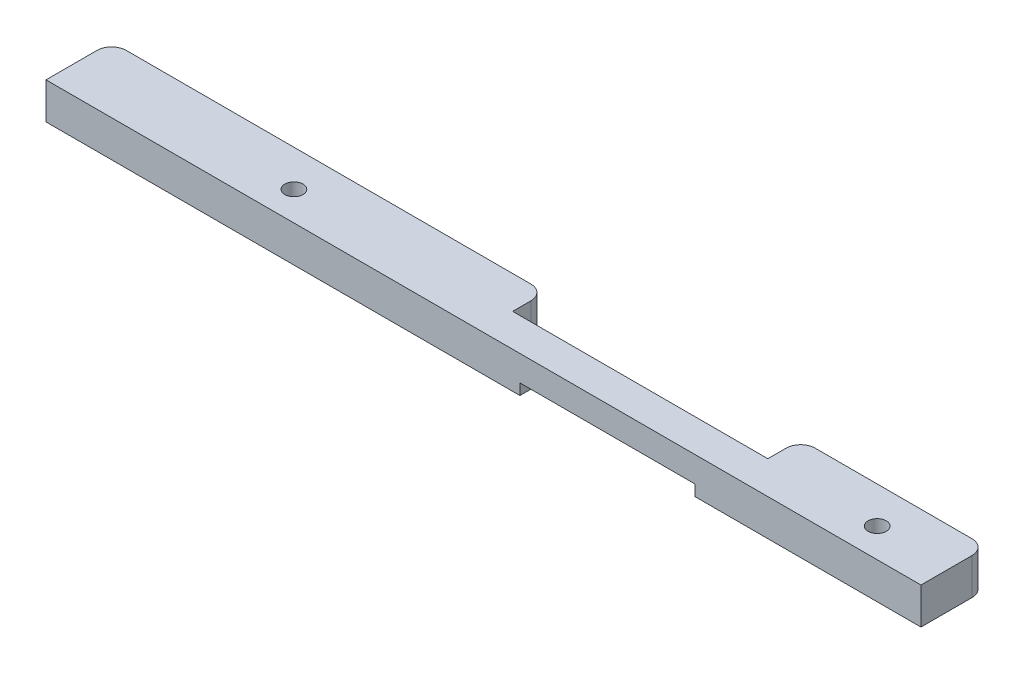
from build123d import *

# Parameters (mm, degrees)
SKETCH1_W             = 120
SKETCH1_H             = 9
BOSS_EXTRUDE1_DEPTH   = 5
M3_TAPPED_HOLE1_D     = 2.5
M3_TAPPED_HOLE1_DEPTH = 8.5
FILLET1_R             = 2
SKETCH4_W             = 35
SKETCH4_H             = 4.5
CUT_EXTRUDE1_DEPTH    = 121.440856855
FILLET2_R             = 2
SKETCH5_W             = 24
SKETCH5_H             = 9
CUT_EXTRUDE2_DEPTH    = 1.5


with BuildPart() as part:
    # Sketch1 → Boss-Extrude1 (new body)
    with BuildSketch(Plane(origin=(0, 0, 0), x_dir=(1, 0, 0), z_dir=(0, 1, 0))):
        with Locations((60, 4.5)):
            Rectangle(SKETCH1_W, SKETCH1_H)
    extrude(amount=BOSS_EXTRUDE1_DEPTH)

    # M3 Tapped Hole1
    with Locations(Plane(origin=(0, 5, 0), x_dir=(-1, 0, 0), z_dir=(0, 1, 0))):
        with Locations((-30, -4), (-110, -4)):
            Hole(M3_TAPPED_HOLE1_D / 2, depth=M3_TAPPED_HOLE1_DEPTH)

    # Fillet1
    fillet1_edges = [part.edges().sort_by_distance(p)[0] for p in [
        (0, 2.5, -9),
        (120, 2.5, -9),
    ]]
    fillet(fillet1_edges, radius=FILLET1_R)

    # Sketch4 → Cut-Extrude1 (cut, through all)
    with BuildSketch(Plane(origin=(0, 5, 0), x_dir=(-1, 0, 0), z_dir=(0, 1, 0))):
        with Locations((-77, -6.75)):
            Rectangle(SKETCH4_W, SKETCH4_H)
    extrude(amount=-CUT_EXTRUDE1_DEPTH, mode=Mode.SUBTRACT)

    # Fillet2
    fillet2_edges = [part.edges().sort_by_distance(p)[0] for p in [
        (94.5, 2.5, -9),
        (59.5, 2.5, -9),
    ]]
    fillet(fillet2_edges, radius=FILLET2_R)

    # Sketch5 → Cut-Extrude2 (cut)
    with BuildSketch(Plane.XZ):
        with Locations((77, -4.5)):
            Rectangle(SKETCH5_W, SKETCH5_H)
    extrude(amount=-CUT_EXTRUDE2_DEPTH, mode=Mode.SUBTRACT)


solid = part.part
